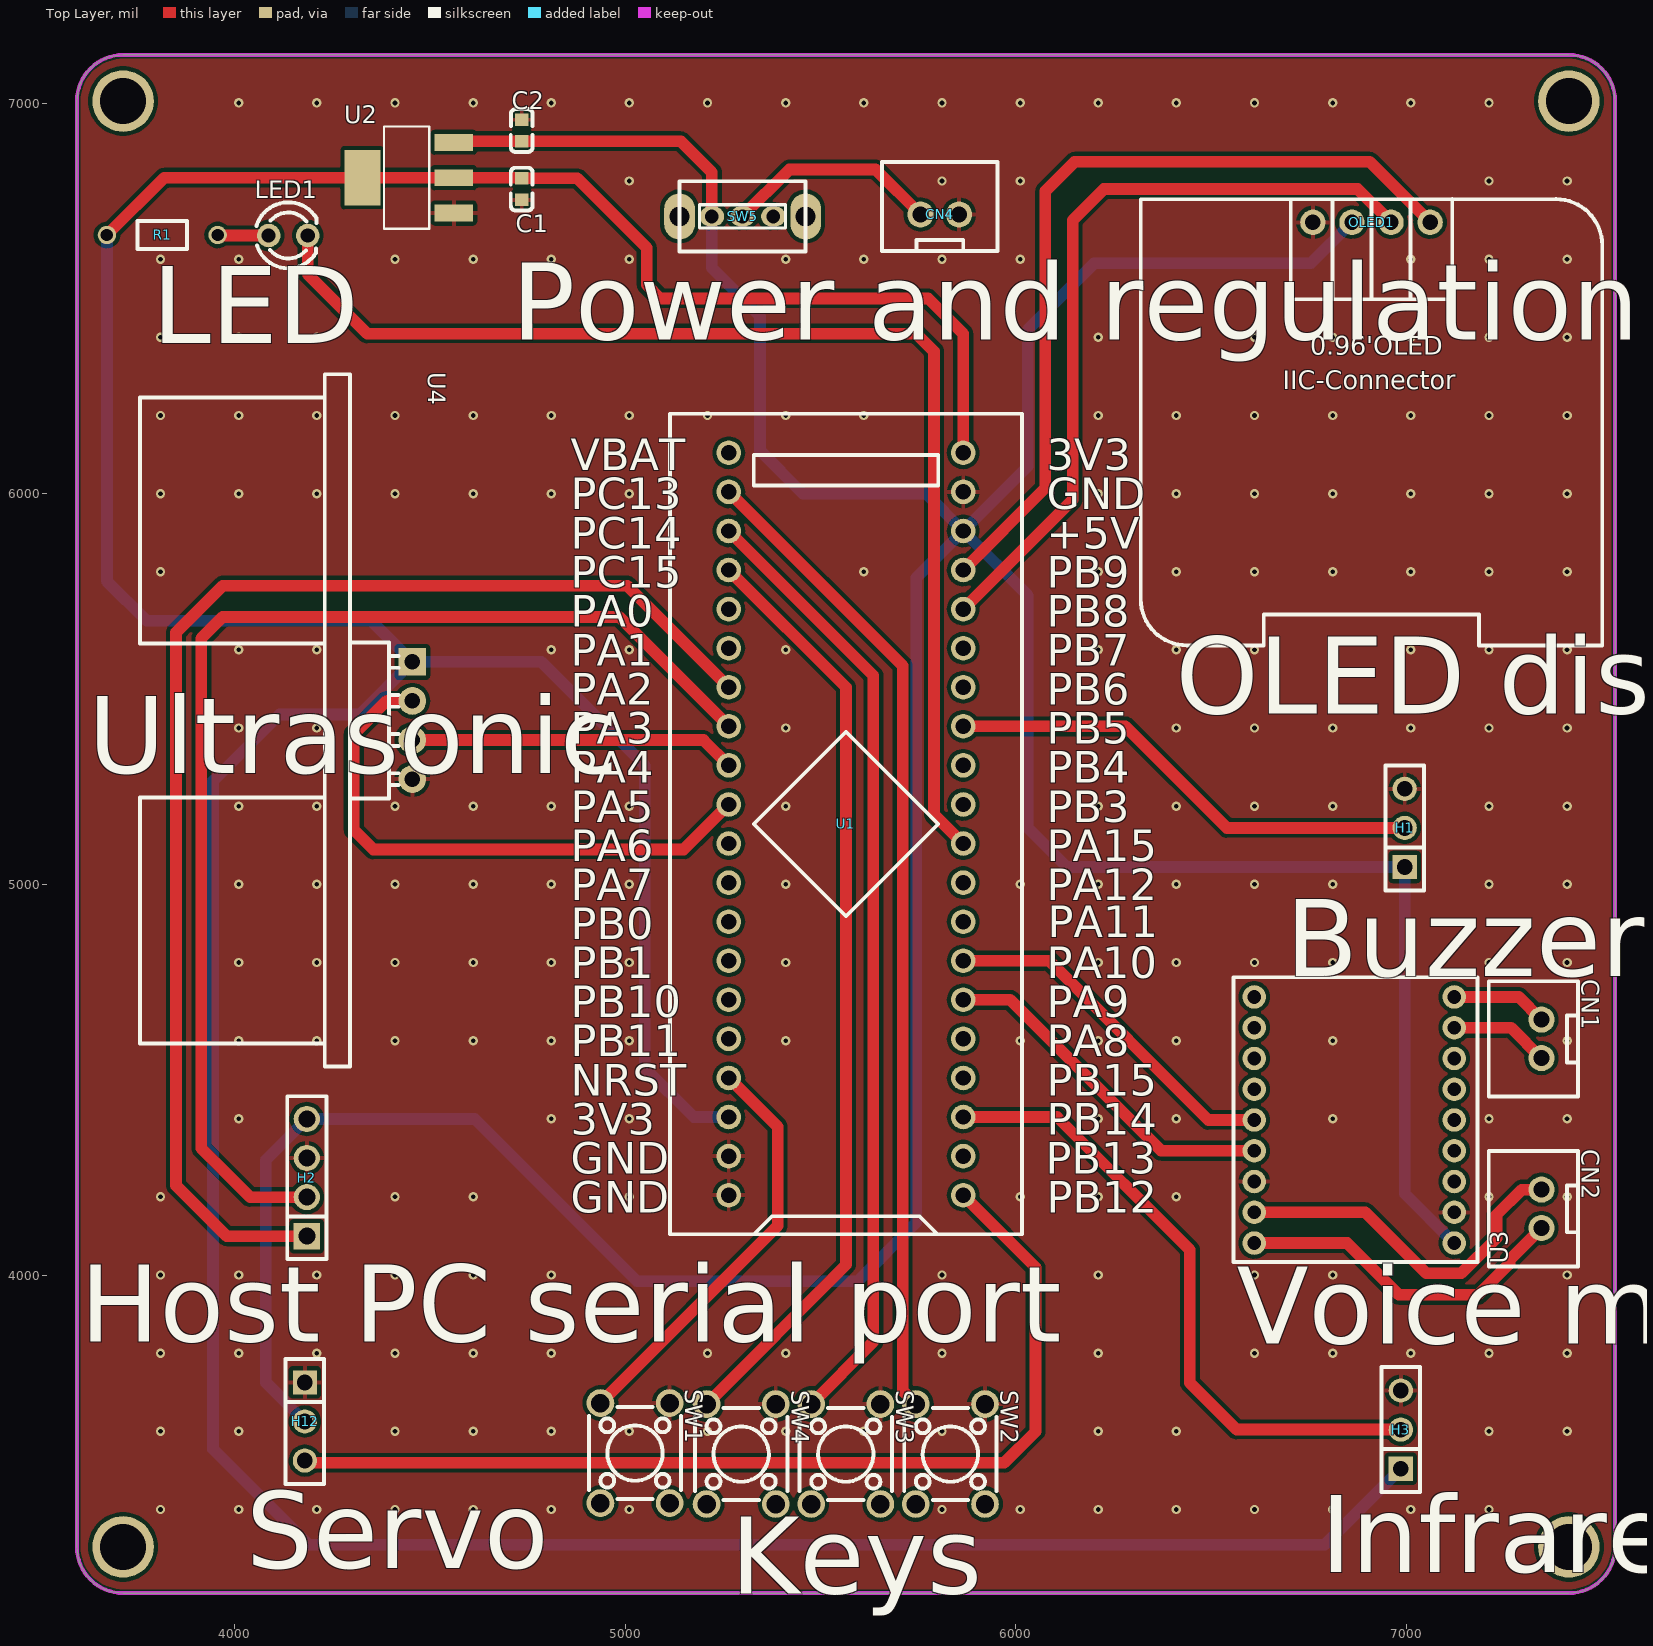
[diagram p0: Top Layer view]
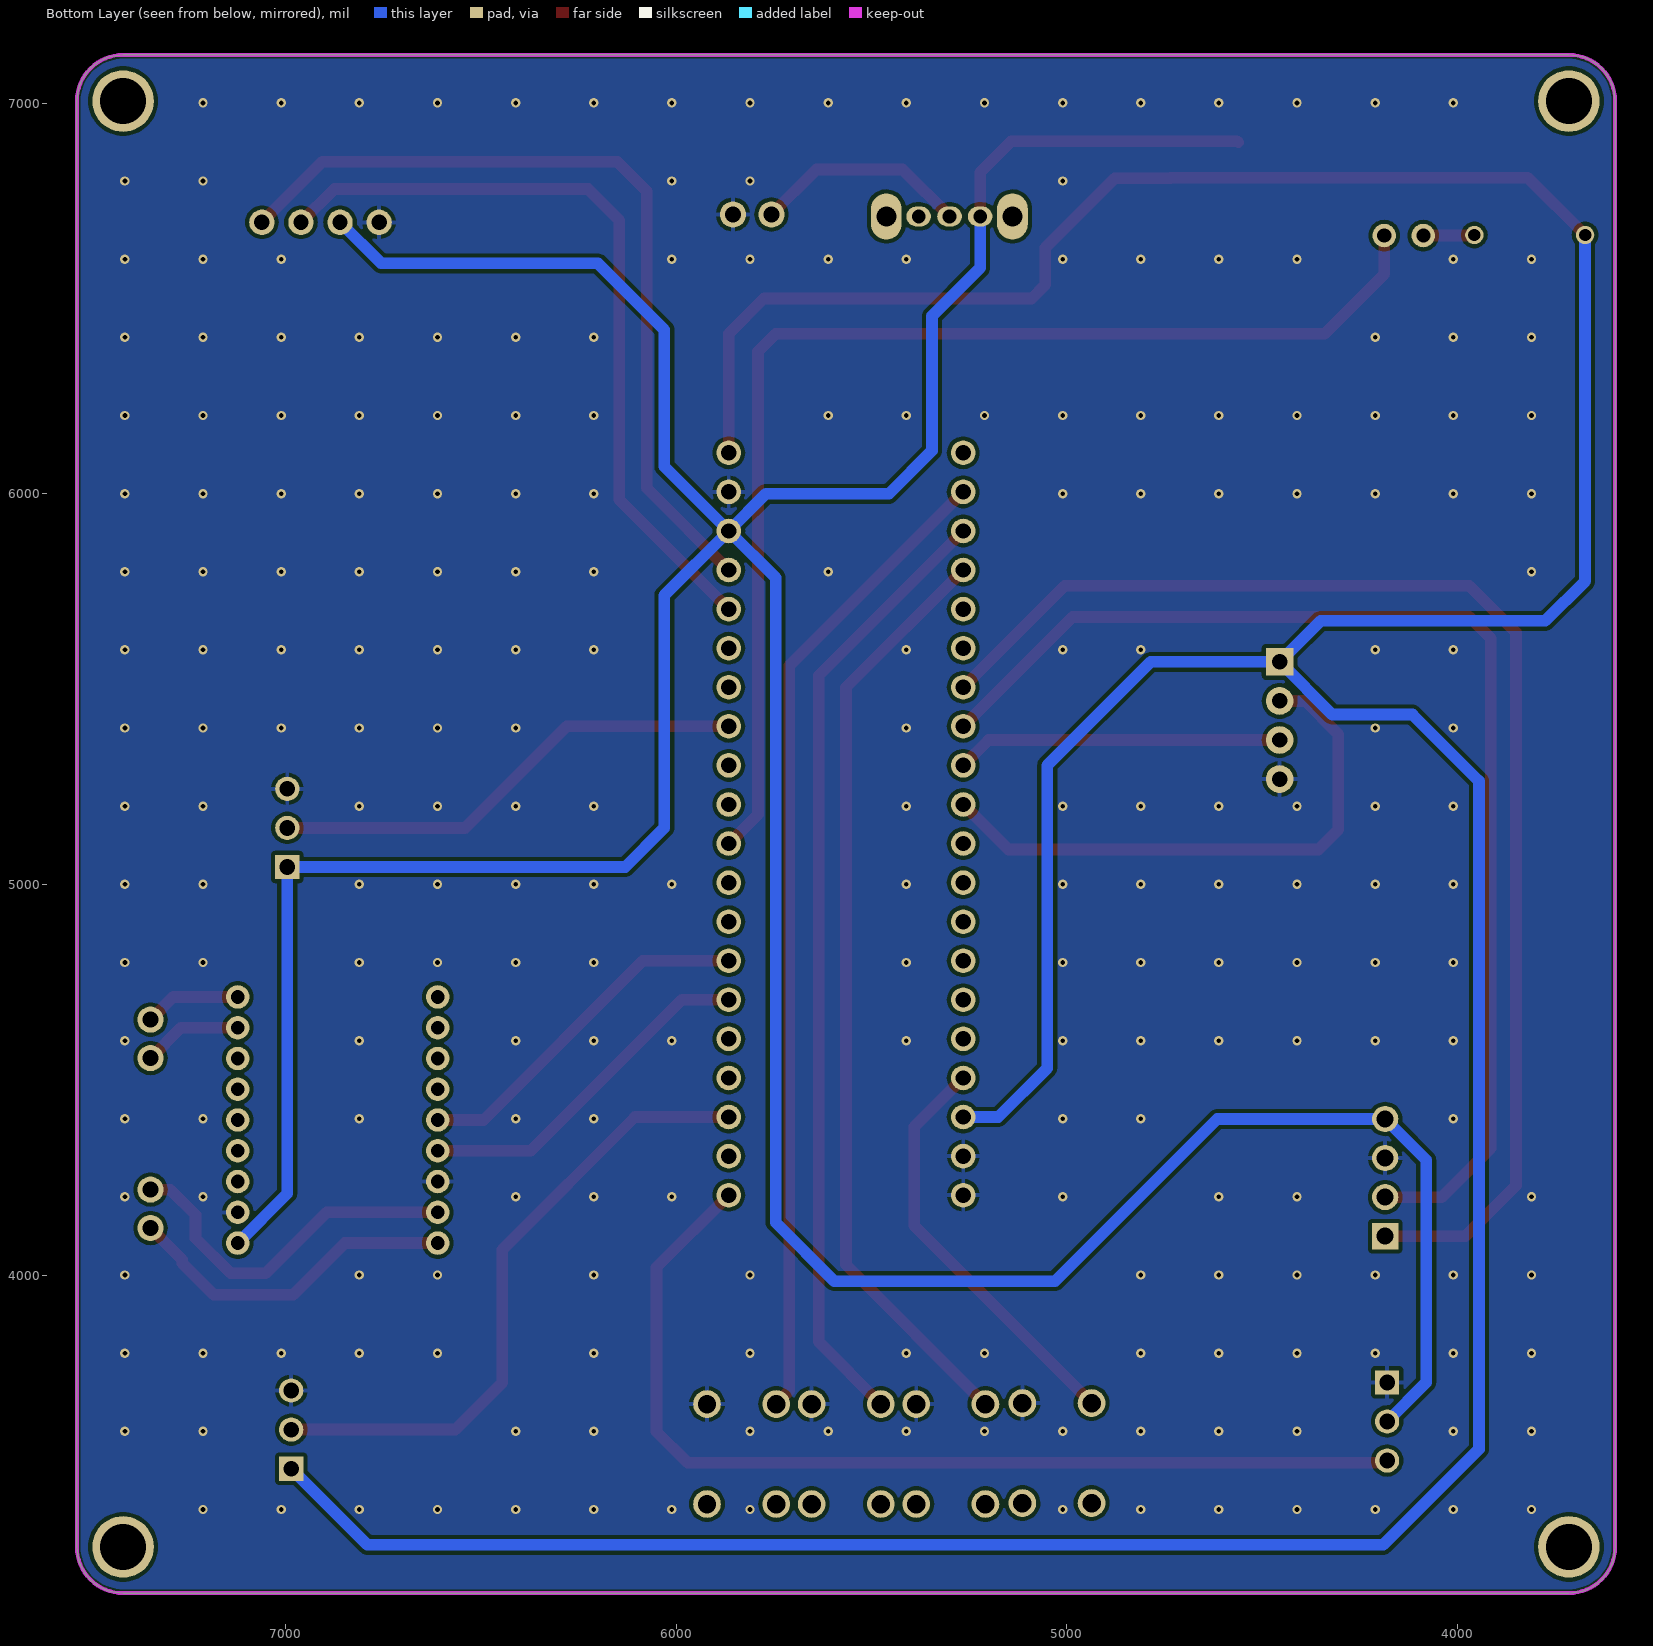
[diagram p1: Bottom Layer view, seen from below]
# Altium PCB MISC89011.pcbdoc
Units mil, origin at the board's own origin, x right, y up, seen from the top; angles counter-clockwise.
Board outline 3937.01 x 3937.01 mil, 2 copper layers (Top Layer, Bottom Layer), stack 62.206 mil thick; 21 components, 43 nets, 122 pads, 230 vias.

## Layer stack, top to bottom
Top Solder Mask Layer: solder mask 0.394, Dk 3.3
Top Layer: signal copper 1.379
Dielectric1: surface 59.449, FR4, Dk 4.5
Bottom Layer: signal copper 1.378
Bottom Solder Mask Layer: solder mask 0.394, Dk 3.3

## Board outline
3714.61,7123.5 ccw(c3714.61,7005.39) 3596.5,7005.39 3596.5,3304.61 ccw(c3714.61,3304.61) 3714.61,3186.5 7415.39,3186.5 ccw(c7415.39,3304.61) 7533.5,3304.61 7533.5,7005.39 ccw(c7415.39,7005.39) 7415.39,7123.5 3714.61,7123.5

## Design rules (kind name [scope] priority, off if disabled: settings)
BoardOutlineClearance copperThickness2oz_1 [All] p2 off: genericclearance=7.99 ignorepadtopadclearanceinfootprint=FALSE except(0: Arc-SplitContinuation Track-SplitContinuation SMDPad-SplitContinuation THPad-SplitContinuation Via-SplitContinuation Fill-SplitContinuation Region-SplitContinuation Poly-SplitContinuation Text-SplitContinuation Hole-SplitContinuation; 5.98: Arc-CutoutEdge Track-CutoutEdge SMDPad-CutoutEdge THPad-CutoutEdge Via-CutoutEdge Text-CutoutEdge; 6.9: Hole-OutlineEdge Hole-CutoutEdge; 10: Poly-OutlineEdge Poly-CutoutEdge; 11.81: Arc-OutlineEdge Track-OutlineEdge SMDPad-OutlineEdge THPad-OutlineEdge Via-OutlineEdge Fill-OutlineEdge Region-OutlineEdge Text-OutlineEdge Fill-CutoutEdge Region-CutoutEdge)
BoardOutlineClearance Plane_innerPlane_1 [All] p4 off: genericclearance=4.02 ignorepadtopadclearanceinfootprint=FALSE except(0: Arc-SplitContinuation Track-SplitContinuation SMDPad-SplitContinuation THPad-SplitContinuation Via-SplitContinuation Fill-SplitContinuation Region-SplitContinuation Poly-SplitContinuation Text-SplitContinuation Hole-SplitContinuation; 5.98: Arc-CutoutEdge Track-CutoutEdge SMDPad-CutoutEdge THPad-CutoutEdge Via-CutoutEdge Text-CutoutEdge; 6.9: Hole-OutlineEdge Hole-CutoutEdge; 10: Poly-OutlineEdge Poly-CutoutEdge; 11.81: Arc-OutlineEdge Track-OutlineEdge SMDPad-OutlineEdge THPad-OutlineEdge Via-OutlineEdge Fill-OutlineEdge Region-OutlineEdge Text-OutlineEdge Fill-CutoutEdge Region-CutoutEdge)
BoardOutlineClearance Copper_copperRegion_1 [All] p6 off: genericclearance=4.02 ignorepadtopadclearanceinfootprint=FALSE except(0: Arc-SplitContinuation Track-SplitContinuation SMDPad-SplitContinuation THPad-SplitContinuation Via-SplitContinuation Fill-SplitContinuation Region-SplitContinuation Poly-SplitContinuation Text-SplitContinuation Hole-SplitContinuation; 5.98: Arc-CutoutEdge Track-CutoutEdge SMDPad-CutoutEdge THPad-CutoutEdge Via-CutoutEdge Text-CutoutEdge; 6.9: Hole-OutlineEdge Hole-CutoutEdge; 10: Poly-OutlineEdge Poly-CutoutEdge; 11.81: Arc-OutlineEdge Track-OutlineEdge SMDPad-OutlineEdge THPad-OutlineEdge Via-OutlineEdge Fill-OutlineEdge Region-OutlineEdge Text-OutlineEdge Fill-CutoutEdge Region-CutoutEdge)
BoardOutlineClearance copperThickness1oz_1 [All] p8: genericclearance=4.02 ignorepadtopadclearanceinfootprint=FALSE except(0: Arc-SplitContinuation Track-SplitContinuation SMDPad-SplitContinuation THPad-SplitContinuation Via-SplitContinuation Fill-SplitContinuation Region-SplitContinuation Poly-SplitContinuation Text-SplitContinuation Hole-SplitContinuation; 5.98: Arc-CutoutEdge Track-CutoutEdge SMDPad-CutoutEdge THPad-CutoutEdge Via-CutoutEdge Text-CutoutEdge; 6.9: Hole-OutlineEdge Hole-CutoutEdge; 10: Poly-OutlineEdge Poly-CutoutEdge; 11.81: Arc-OutlineEdge Track-OutlineEdge SMDPad-OutlineEdge THPad-OutlineEdge Via-OutlineEdge Fill-OutlineEdge Region-OutlineEdge Text-OutlineEdge Fill-CutoutEdge Region-CutoutEdge)
Clearance copperThickness2oz [All] p1 off: gap=7.99 ignorepadtopadclearanceinfootprint=FALSE except(5.98: SMDPad-Track SMDPad-SMDPad THPad-Track SMDPad-THPad THPad-THPad Track-Via SMDPad-Via THPad-Via Via-Via Fill-SMDPad Region-SMDPad Fill-THPad Region-THPad Fill-Via Region-Via Fill-Fill Fill-Region Region-Region Arc-Track Arc-SMDPad Arc-THPad Arc-Via Fill-Arc Region-Arc Arc-Arc Text-Track SMDPad-Text Text-THPad Text-Via Fill-Text Region-Text Arc-Text Text-Text; 6.9: Hole-Track Hole-SMDPad Hole-THPad Hole-Via Fill-Hole Region-Hole Hole-Arc Hole-Text; 10: Poly-Track Poly-SMDPad Poly-THPad Poly-Via Poly-Fill Poly-Region Poly-Poly Poly-Arc Poly-Text Poly-Hole; 11.81: Fill-Track Region-Track)
Clearance Plane_innerPlane [All] p3 off: gap=4.02 ignorepadtopadclearanceinfootprint=FALSE except(5.98: SMDPad-Track SMDPad-SMDPad THPad-Track SMDPad-THPad THPad-THPad Track-Via SMDPad-Via THPad-Via Via-Via Fill-SMDPad Region-SMDPad Fill-THPad Region-THPad Fill-Via Region-Via Fill-Fill Fill-Region Region-Region Arc-Track Arc-SMDPad Arc-THPad Arc-Via Fill-Arc Region-Arc Arc-Arc Text-Track SMDPad-Text Text-THPad Text-Via Fill-Text Region-Text Arc-Text Text-Text; 6.9: Hole-Track Hole-SMDPad Hole-THPad Hole-Via Fill-Hole Region-Hole Hole-Arc Hole-Text; 10: Poly-Track Poly-SMDPad Poly-THPad Poly-Via Poly-Fill Poly-Region Poly-Poly Poly-Arc Poly-Text Poly-Hole; 11.81: Fill-Track Region-Track)
Clearance Copper_copperRegion [All] p5 off: gap=4.02 ignorepadtopadclearanceinfootprint=FALSE except(5.98: SMDPad-Track SMDPad-SMDPad THPad-Track SMDPad-THPad THPad-THPad Track-Via SMDPad-Via THPad-Via Via-Via Fill-SMDPad Region-SMDPad Fill-THPad Region-THPad Fill-Via Region-Via Fill-Fill Fill-Region Region-Region Arc-Track Arc-SMDPad Arc-THPad Arc-Via Fill-Arc Region-Arc Arc-Arc Text-Track SMDPad-Text Text-THPad Text-Via Fill-Text Region-Text Arc-Text Text-Text; 6.9: Hole-Track Hole-SMDPad Hole-THPad Hole-Via Fill-Hole Region-Hole Hole-Arc Hole-Text; 10: Poly-Track Poly-SMDPad Poly-THPad Poly-Via Poly-Fill Poly-Region Poly-Poly Poly-Arc Poly-Text Poly-Hole; 11.81: Fill-Track Region-Track)
Clearance copperThickness1oz [All] p7: gap=4.02 ignorepadtopadclearanceinfootprint=FALSE except(5.98: SMDPad-Track SMDPad-SMDPad THPad-Track SMDPad-THPad THPad-THPad Track-Via SMDPad-Via THPad-Via Via-Via Fill-SMDPad Region-SMDPad Fill-THPad Region-THPad Fill-Via Region-Via Fill-Fill Fill-Region Region-Region Arc-Track Arc-SMDPad Arc-THPad Arc-Via Fill-Arc Region-Arc Arc-Arc Text-Track SMDPad-Text Text-THPad Text-Via Fill-Text Region-Text Arc-Text Text-Text; 6.9: Hole-Track Hole-SMDPad Hole-THPad Hole-Via Fill-Hole Region-Hole Hole-Arc Hole-Text; 10: Poly-Track Poly-SMDPad Poly-THPad Poly-Via Poly-Fill Poly-Region Poly-Poly Poly-Arc Poly-Text Poly-Hole; 11.81: Fill-Track Region-Track)
DiffPairsRouting differentialPair [All] p1: maxlimit=6 minlimit=6 mostfreqgap=6 toplayer_minwidth=5 toplayer_prefwidth=10 toplayer_maxwidth=100 toplayer_mingap=6 toplayer_prefgap=6 toplayer_maxgap=6 bottomlayer_minwidth=5 bottomlayer_prefwidth=10 bottomlayer_maxwidth=100 bottomlayer_mingap=6 bottomlayer_prefgap=6 bottomlayer_maxgap=6 maxuncoupledlength=10
HoleToHoleClearance otherClearance [All] p1: gap=11.81 allowstackedmicrovias=TRUE
Length netLength [All] p1: minlimit=0 maxlimit=0
PasteMaskExpansion pasteMaskExpansion [All] p1: expansion=0
PlaneConnect innerPlane [All] p1: planeconnectstyle=Relief reliefexpansion=20 reliefentries=4 reliefconductorwidth=10 reliefairgap=10
PolygonConnect copperRegion [All] p1: connectstyle=Relief reliefconductorwidth=10 reliefentries=4 polygonreliefangle="90 Angle" airgapwidth=10 via.connectstyle=Relief via.reliefconductorwidth=10 via.reliefentries=4 via.polygonreliefangle="90 Angle" via.airgapwidth=10
RoutingVias viaSize [All] p1: holewidth=12.01 width=24.02 viastyle="Through Hole" minholewidth=11.81 minwidth=19.68 maxholewidth=248.03 maxwidth=393.7
SolderMaskExpansion solderMaskExpansion [IsVia] p1: expansion=-1000 istentingtop=TRUE
SolderMaskExpansion solderMaskExpansion [All] p2: expansion=2 istentingtop=FALSE
Width copperThickness2oz_2 [All] p1 off: maxlimit=100 minlimit=8 preferedwidth=10
Width copperThickness1oz_2 [All] p2: maxlimit=100 minlimit=5 preferedwidth=10

## Components (designator, comment, footprint, x,y, rotation, side; value= is the part's Value field where it differs from the comment)
C1 "100nF" C0603 4735,6780 r90 top
C2 "100nF" C0603 4735,6930 r270 top
CN1 "XH2.54*2P_through-hole" CONN-TH_2P-P2.50-XH2.54-2P 7345,4605 r270 top
CN2 "XH2.54*2P_through-hole" CONN-TH_2P-P2.50-XH2.54-2P 7345,4170 r270 top
CN4 "XH2.54*2P_through-hole" CONN-TH_2P-P2.50-XH2.54-2P 5805,6715 r180 top
H1 "" HDR-TH_3P-P2.54-V-F 6995,5145 r90 top
H2 "" HDR-TH_4P-P2.54-V-F 4185,4250 r90 top
H3 "" HDR-TH_3P-P2.54-V-F 6985,3605 r90 top
H12 "" HDR-TH_3P-P2.54-V-F 4180,3625.79 r270 top
LED1 "" LED_TH-3mm 4137.42,6661.15 r0 top
OLED1 "" 0.96OLED_4P 6910,6695 r0 top
R1 "220Ω" Res_1/8W 3815,6665 r180 top
SW1 "" SW-TH_4P-L6.0-W6.0-P4.50-LS6.5 5025,3545 r270 top
SW2 "" SW-TH_4P-L6.0-W6.0-P4.50-LS6.5 5832.14,3542.47 r270 top
SW3 "" SW-TH_4P-L6.0-W6.0-P4.50-LS6.5 5564.43,3542.47 r270 top
SW4 "" SW-TH_4P-L6.0-W6.0-P4.50-LS6.5 5296.72,3542.47 r270 top
SW5 "" 拨动开关 5295,6710 r0 top
U1 "STM32F103C8T6-Card" CONN-TH_L53.3-W22.9_STM32F103C8T6-CARD 5565,5155 r90 top
U2 "AMS1117-3.3" SOT-223-3_L6.5-W3.4-P2.30-LS7.0-BR 4444.33,6809.1 r0 top
U3 "CON2.0MM-PAD-18" CONN-TH_18P-P2.00_C9900078766 7121.85,4397.38 r90 top
U4 "HC-SR04" TH_HC-SR04V 4455,5420 r270 top

## Footprints (in the part's own frame and the unit in brackets; to place one, negate y for a bottom-side part, rotate by r counter-clockwise, add the part's x,y. Pads: shape width x height; smd on the part's side, far side on the other; paste and mask are expansions set on the pad)
0.96OLED_4P [mm]
  round 1.65 hole 1 copper offset 0,0: 1(-3.81,-0.001) 2(-1.27,0.002) 3(1.27,0.002) 4(3.81,0.002)
  silkscreen extent -15,-27.5 15,1.5
C0603 [mm]
  rect 0.8x0.9 smd: 1(-0.7,0) 2(0.7,0)
  silkscreen extent -1.39,-0.71 1.39,0.71
CONN-TH_2P-P2.50-XH2.54-2P [mm]
  round 1.7 hole 1.05 paste+0 mask+0.05: 1(1.25,0) 2(-1.25,0)
  silkscreen extent -3.75,-3.42 3.75,2.37
CONN-TH_18P-P2.00_C9900078766 [mil]
  round 60 hole 35.43 paste+0 mask+1.97: 1(-314.96,0.01) 2(-314.96,511.81) 3(-236.22,0.01) 4(-236.22,511.81) 5(-157.48,0.01) 6(-157.48,511.81) 9(0,0) 10(0,511.81) 11(78.74,0) 12(78.74,511.81) 13(157.48,0) 14(157.48,511.81) 15(236.22,0) 16(236.22,511.81) 17(314.96,0) 18(314.96,511.81)
  round 60 hole 35.43 copper offset -0.01,0 paste+0 mask+1.97: 7(-78.72,0.01) 8(-78.72,511.81)
  silkscreen extent -363,-60 365,565
CONN-TH_L53.3-W22.9_STM32F103C8T6-CARD [mm]
  round 1.6 hole 1: 1(-24.13,-7.62) 2(-21.59,-7.62) 3(-19.05,-7.62) 4(-16.51,-7.62) 5(-13.97,-7.62) 6(-11.43,-7.62) 7(-8.89,-7.62) 8(-6.35,-7.62) 9(-3.81,-7.62) 10(-1.27,-7.62) 11(1.27,-7.62) 12(3.81,-7.62) 13(6.35,-7.62) 14(8.89,-7.62) 15(11.43,-7.62) 16(13.97,-7.62) 17(16.51,-7.62) 18(19.05,-7.62) 19(21.59,-7.62) 20(24.13,-7.62) 21(24.13,7.62) 22(21.59,7.62) 23(19.05,7.62) 24(16.51,7.62) 25(13.97,7.62) 26(11.43,7.62) 27(8.89,7.62) 28(6.35,7.62) 29(3.81,7.62) 30(1.27,7.62) 31(-1.27,7.62) 32(-3.81,7.62) 33(-6.35,7.62) 34(-8.89,7.62) 35(-11.43,7.62) 36(-13.97,7.62) 37(-16.51,7.62) 38(-19.05,7.62) 39(-21.59,7.62) 40(-24.13,7.62)
  silkscreen extent -26.67,-11.43 26.67,11.43
HDR-TH_3P-P2.54-V-F [mil]
  rect 62x62 hole 40.16: 1(-100,0)
  round 62 hole 40.16: 2(0,0) 3(100,0)
  silkscreen extent -160,-49 160,49
HDR-TH_4P-P2.54-V-F [mm]
  rect 1.7x1.7 hole 1.1: 1(-3.81,0)
  round 1.7 hole 1.1: 2(-1.27,0) 3(1.27,0) 4(3.81,0)
  silkscreen extent -5.29,-1.27 5.29,1.27
LED_TH-3mm [mil]
  round 60 hole 36 paste+0 mask+2: 1(-50,0) 2(50,0)
  silkscreen extent -81,-84 72,85
Res_1/8W [mil]
  round 47.2 hole 31.5 paste+0 mask+2: 1(-141.7,2.48) 2(141.7,2.48)
  silkscreen extent -63,-33 63,38
SOT-223-3_L6.5-W3.4-P2.30-LS7.0-BR [mm]
  rect 2.5x1.1 smd: 1(2.97,-2.3) 2(2.97,0) 3(2.97,2.3)
  rect 2.34x3.6 smd: 4(-2.97,0)
  silkscreen extent -1.57,-3.33 1.37,3.33
SW-TH_4P-L6.0-W6.0-P4.50-LS6.5 [mm]
  round 1.8 hole 1.2: 1(-3.25,2.25) 2(3.25,2.25) 3(-3.25,-2.25) 4(3.25,-2.25)
  silkscreen extent -3,-3 3,3
TH_HC-SR04V [mm]
  rect 1.8x1.8 hole 1.001: 1(-3.81,0)
  round 1.8 hole 1.001: 2(-1.27,0) 3(1.27,0) 4(3.81,0)
  silkscreen extent -22.5,-17.7 22.5,-0.89
拨动开关 [mil]
  oval 63x51.2 hole 35.4 paste+0 mask+2: 1(-73.4,0) 2(5,0) 3(84,0)
  oval 78.7x118.1 hole 51.2 paste+0 mask+2: 4(166.7,0) 5(-156.1,0)
  silkscreen extent -156,-90 167,90

## Free pads (board coordinates)
  round 157.48 hole 118.11: 1(3714.61,7005.39) 1(3714.61,3304.61) 1(7415.39,7005.39) 1(7415.39,3304.61)

## Via types
v1: diameter 24.02, hole 12, Top Layer to Bottom Layer, 230 vias

## Nets (pads, with @x,y where several pads share a name; then routed paths per layer and width w, separated by ;. In a path a pad name is that pad's centre, name@x,y a point inside that pad or via, vN(x,y) a via of type N, cw(c..) or ccw(c..) an arc to the next point about the centre after c; other vN are vias at no path point)
$1N17118: CN4.1 SW5.2 | length 553.1
  Top Layer w30: SW5.2 5420,6830 5640.78,6830 CN4.1
$1N17153: LED1.1 R1.1 | length 131.3
  Top Layer w30: R1.1 3958.08,6661.15 LED1.1
+5V: C2.2 H1.1 H2.4 H12.2 OLED1.2 SW5.1 U1.18 U2.3 U3.1 | length 10913.7
  Top Layer w30: U2.3 4564.05,6902.44 C2.2 5142.56,6902.44 5221.6,6823.4 SW5.1
  Bottom Layer w30: H12.2 4080,3725.79 4080,4295 H2.4 4615,4400 5030,3985 5595,3985 5745,4135 5745,5785 U1.18 ; SW5.1 5221.6,6578.4 5345,6455 5345,6110 5455,6000 5770,6000 U1.18 ; OLED1.2@6860,6695.05 6754.95,6590 6200,6590 6030,6420 6030,6070 U1.18 ; U3.1 6995,4209.26 H1.1 6130,5045 6030,5145 6030,5740 U1.18
GND: C1.1 C2.1 CN4.2 H1.3 H2.3 H3.3 H12.1 OLED1.1 SW1.1 SW2.1 SW3.1 SW4.1 U1.19 U1.39 U1.40 U2.1 U3.3 U3.6 U4.4
  other v1: 3810.6,3400.6 4010.6,3400.6 4210.6,3400.6 4410.6,3400.6 4610.6,3400.6 4810.6,3400.6 5010.6,3400.6 5810.6,3400.6 6010.6,3400.6 6210.6,3400.6 6410.6,3400.6 6610.6,3400.6 6810.6,3400.6 7010.6,3400.6 7210.6,3400.6 3810.6,3600.6 4010.6,3600.6 4410.6,3600.6 4610.6,3600.6 4810.6,3600.6 5010.6,3600.6 5210.6,3600.6 5410.6,3600.6 5610.6,3600.6 5810.6,3600.6 6210.6,3600.6 6410.6,3600.6 7210.6,3600.6 7410.6,3600.6 3810.6,3800.6 4010.6,3800.6 4210.6,3800.6 4410.6,3800.6 4610.6,3800.6 4810.6,3800.6 5210.6,3800.6 5410.6,3800.6 5810.6,3800.6 6210.6,3800.6 6610.6,3800.6 6810.6,3800.6 7010.6,3800.6 7210.6,3800.6 7410.6,3800.6 3810.6,4000.6 4010.6,4000.6 4210.6,4000.6 4410.6,4000.6 4610.6,4000.6 4810.6,4000.6 5810.6,4000.6 6210.6,4000.6 6610.6,4000.6 6810.6,4000.6 7410.6,4000.6 3810.6,4200.6 4410.6,4200.6 4610.6,4200.6 5010.6,4200.6 6010.6,4200.6 6210.6,4200.6 6410.6,4200.6 7210.6,4200.6 7410.6,4200.6 4010.6,4400.6 4810.6,4400.6 5010.6,4400.6 6210.6,4400.6 6410.6,4400.6 6810.6,4400.6 7210.6,4400.6 7410.6,4400.6 4010.6,4600.6 4210.6,4600.6 4410.6,4600.6 4610.6,4600.6 4810.6,4600.6 5010.6,4600.6 5410.6,4600.6 6010.6,4600.6 6210.6,4600.6 6410.6,4600.6 6810.6,4600.6 7410.6,4600.6 4010.6,4800.6 4210.6,4800.6 4410.6,4800.6 4610.6,4800.6 4810.6,4800.6 5010.6,4800.6 5410.6,4800.6 6210.6,4800.6 6410.6,4800.6 6610.6,4800.6 6810.6,4800.6 7210.6,4800.6 7410.6,4800.6 4010.6,5000.6 4210.6,5000.6 4410.6,5000.6 4610.6,5000.6 4810.6,5000.6 5010.6,5000.6 5410.6,5000.6 6010.6,5000.6 6210.6,5000.6 6410.6,5000.6 6610.6,5000.6 6810.6,5000.6 7210.6,5000.6 7410.6,5000.6 4010.6,5200.6 4210.6,5200.6 4410.6,5200.6 4610.6,5200.6 4810.6,5200.6 5010.6,5200.6 5410.6,5200.6 6210.6,5200.6 6410.6,5200.6 6610.6,5200.6 6810.6,5200.6 7210.6,5200.6 7410.6,5200.6 4010.6,5400.6 4210.6,5400.6 5410.6,5400.6 6410.6,5400.6 6610.6,5400.6 6810.6,5400.6 7010.6,5400.6 7210.6,5400.6 7410.6,5400.6 4010.6,5600.6 4210.6,5600.6 4810.6,5600.6 5010.6,5600.6 5410.6,5600.6 6210.6,5600.6 6410.6,5600.6 6610.6,5600.6 6810.6,5600.6 7010.6,5600.6 7210.6,5600.6 7410.6,5600.6 3810.6,5800.6 5610.6,5800.6 6210.6,5800.6 6410.6,5800.6 6610.6,5800.6 6810.6,5800.6 7010.6,5800.6 7210.6,5800.6 7410.6,5800.6 3810.6,6000.6 4010.6,6000.6 4210.6,6000.6 4410.6,6000.6 4610.6,6000.6 4810.6,6000.6 5010.6,6000.6 6210.6,6000.6 6410.6,6000.6 6610.6,6000.6 6810.6,6000.6 7010.6,6000.6 7210.6,6000.6 7410.6,6000.6 3810.6,6200.6 4010.6,6200.6 4210.6,6200.6 4410.6,6200.6 4610.6,6200.6 4810.6,6200.6 5010.6,6200.6 5210.6,6200.6 5410.6,6200.6 5610.6,6200.6 6210.6,6200.6 6410.6,6200.6 6610.6,6200.6 6810.6,6200.6 7010.6,6200.6 7210.6,6200.6 7410.6,6200.6 3810.6,6400.6 4010.6,6400.6 4210.6,6400.6 6210.6,6400.6 6410.6,6400.6 6610.6,6400.6 6810.6,6400.6 7010.6,6400.6 7210.6,6400.6 7410.6,6400.6 3810.6,6600.6 4010.6,6600.6 4410.6,6600.6 4610.6,6600.6 4810.6,6600.6 5010.6,6600.6 5410.6,6600.6 5610.6,6600.6 5810.6,6600.6 6010.6,6600.6 7010.6,6600.6 7210.6,6600.6 7410.6,6600.6 5010.6,6800.6 5810.6,6800.6 6010.6,6800.6 7210.6,6800.6 7410.6,6800.6 4010.6,7000.6 4210.6,7000.6 4410.6,7000.6 4610.6,7000.6 4810.6,7000.6 5010.6,7000.6 5210.6,7000.6 5410.6,7000.6 5610.6,7000.6 5810.6,7000.6 6010.6,7000.6 6210.6,7000.6 6410.6,7000.6 6610.6,7000.6 6810.6,7000.6 7010.6,7000.6 7210.6,7000.6
MIC+: CN1.1 U3.15 | length 255.4
  Top Layer w30: U3.15@7121.85,4633.6 7267.19,4633.6 CN1.1
MIC-: CN1.2 U3.17 | length 247.2
  Top Layer w30: U3.17@7121.85,4712.34 7286.88,4712.34 CN1.2
NRST: SW1.3 U1.37 | length 1071.7
  Top Layer w30: SW1.3 5390,4126.53 5390,4380 U1.37
PA0: U1.25
PA1: U1.26
PA2: H2.1 U1.27 | length 3376.2
  Top Layer w30: H2.1 3980,4100 3850,4230 3850,5645 3970,5765 5005,5765 U1.27
PA3: H2.2 U1.28 | length 3115.5
  Top Layer w30: H2.2 4040,4200 3915,4325 3915,5630 3970,5685 4985,5685 U1.28
PA4: U1.29 U4.3 | length 836.9
  Top Layer w30: U4.3 5200,5370 U1.29
PA5: U1.30 U4.2 | length 1458.6
  Top Layer w30: U4.2 4390,5470 4305,5385 4305,5140 4355,5090 5150,5090 U1.30
PA6: U1.31
PA7: U1.32
PA8: U1.5
PA9: U1.6 U3.8 | length 905.1
  Top Layer w30: U1.6 5985,4705 6371.35,4318.65 U3.8@6610.04,4318.65
PA10: U1.7 U3.10 | length 913.9
  Top Layer w30: U1.7 6085,4805 6492.62,4397.38 U3.10
PA11: U1.8
PA12: U1.9
PA15: LED1.2 U1.10 | length 3074.1
  Top Layer w30: LED1.2 4187.42,6562.58 4340,6410 5745,6410 5790,6365 5790,5180 U1.10
PB0: U1.33
PB1: U1.34
PB3: U1.11
PB4: U1.12
PB5: H1.2 U1.13 | length 1237.7
  Top Layer w30: U1.13 6280,5405 6540,5145 H1.2
PB6: U1.14
PB7: U1.15
PB8: OLED1.3 U1.16 | length 1994.3
  Top Layer w30: U1.16 6145,5985 6145,6700 6225,6780 6875.05,6780 OLED1.3@6960,6695.05
PB9: OLED1.4 U1.17 | length 2137.2
  Top Layer w30: U1.17 6075,6015 6075,6775 6150,6850 6905.05,6850 OLED1.4@7060,6695.05
PB10: U1.35
PB11: U1.36
PB12: H12.3 U1.1 | length 2587.2
  Top Layer w30: H12.3 4185.79,3520 5970,3520 6050,3600 6050,4020 U1.1
PB13: U1.2
PB14: H3.2 U1.3 | length 1650.5
  Top Layer w30: U1.3 6105,4405 6445,4065 6445,3725 6565,3605 H3.2
PB15: U1.4
PC13: SW2.3 U1.22 | length 2532.8
  Top Layer w30: U1.22 5710,5560 5710,3703.98 SW2.3
PC14: SW3.3 U1.23 | length 2453.8
  Top Layer w30: U1.23 5635,5535 5635,3829.57 SW3.3
PC15: SW4.3 U1.24 | length 2406.7
  Top Layer w30: SW4.3 5565,4027.28 5565,5505 U1.24
SPK+: CN2.1 U3.2 | length 865.8
  Top Layer w30: U3.2 6847.58,4082.42 6980,3950 7183.11,3950 7264.02,4030.91 7264.02,4039.8 CN2.1
SPK-: CN2.2 U3.4 | length 923.5
  Top Layer w30: U3.4 6893.84,4161.16 7050,4005 7140,4005 7230,4095 7230,4155 7294.22,4219.22 CN2.2
VBAT: U1.21
VCC: C1.2 H3.1 R1.2 U1.20 U1.38 U2.2 U2.4 U4.1 | length 11846.6
  Top Layer w30: R1.2 3819.87,6809.1 U2.4 U2.2 4733.46,6809.1 C1.2 4877.44,6807.56 5055,6630 5055,6535 5090,6500 5775,6500 5865,6410 U1.20
  Bottom Layer w30: R1.2 3673.3,5776.7 3775,5675 4350,5675 U4.1 ; U1.38 5175,4405 5050,4530 5050,5305 4785,5570 U4.1 ; H3.1 6790,3310 4190,3310 3945,3555 3945,5265 4115,5435 4320,5435 U4.1
pads on no net: SW1.2 SW1.4 SW2.2 SW2.4 SW3.2 SW3.4 SW4.2 SW4.4 SW5.3 SW5.4 SW5.5 U3.5 U3.7 U3.9 U3.11 U3.12 U3.13 U3.14 U3.16 U3.18

## Polygon pours and split planes (outlines as drawn)
GND on Bottom Layer (solid, remove dead copper, pour order 2): 3525,7245 3525,3080 7700,3080 7700,7245
GND on Top Layer (solid, remove dead copper, pour order 2): 3000,7415 3000,3000 7930,3000 7930,7415

## Keep-outs
Board Outline Layer:
  the board outline again, w10

## Silkscreen, mask and mechanical layers (free items; w line width, h text height)
Top Silkscreen Layer:
  text "Power and regulation" at 4710,6395 h196.85
  text "LED" at 3790,6385 h196.85
  text "VBAT" at 4860.95,6060 h80
  text "3V3" at 6079.16,6060 h80
  text "PC13" at 4860.95,5960 h80
  text "GND" at 6079.16,5960 h80
  text "PC14" at 4860.95,5860 h80
  text "+5V" at 6079.16,5860 h80
  text "PC15" at 4860.95,5760 h80
  text "PB9" at 6079.16,5760 h80
  text "PA0" at 4860.95,5660 h80
  text "PB8" at 6079.16,5660 h80
  text "PA1" at 4860.95,5560 h80
  text "PB7" at 6079.16,5560 h80
  text "PA2" at 4860.95,5460 h80
  text "PB6" at 6079.16,5460 h80
  text "OLED display" at 6408.66,5436.57 h196.85
  text "PA3" at 4860.95,5360 h80
  text "PB5" at 6079.16,5360 h80
  text "Ultrasonic" at 3625,5285 h196.85
  text "PA4" at 4860.95,5260 h80
  text "PB4" at 6079.16,5260 h80
  text "PA5" at 4860.95,5160 h80
  text "PB3" at 6079.16,5160 h80
  text "PA6" at 4860.95,5060 h80
  text "PA15" at 6079.16,5060 h80
  text "PA7" at 4860.95,4960 h80
  text "PA12" at 6079.16,4960 h80
  text "PA11" at 6080.95,4865 h80
  text "PB0" at 4860.95,4860 h80
  text "Buzzer" at 6690,4765 h196.85
  text "PB1" at 4860.95,4760 h80
  text "PA10" at 6079.16,4760 h80
  text "PB10" at 4860.95,4660 h80
  text "PA9" at 6079.16,4660 h80
  text "PB11" at 4860.95,4560 h80
  text "PA8" at 6079.16,4560 h80
  text "NRST" at 4860.95,4460 h80
  text "PB15" at 6079.16,4460 h80
  text "3V3" at 4860.95,4360 h80
  text "PB14" at 6079.16,4360 h80
  text "GND" at 4860.95,4260 h80
  text "PB13" at 6075.95,4260 h80
  text "GND" at 4860.95,4160 h80
  text "PB12" at 6079.16,4160 h80
  text "Host PC serial port" at 3605,3830 h196.85
  text "Voice module" at 6565,3825 h196.85
  text "Servo" at 4030,3250 h196.85
  text "Infrared" at 6780,3240 h196.85
  text "Keys" at 5270,3185 h196.85